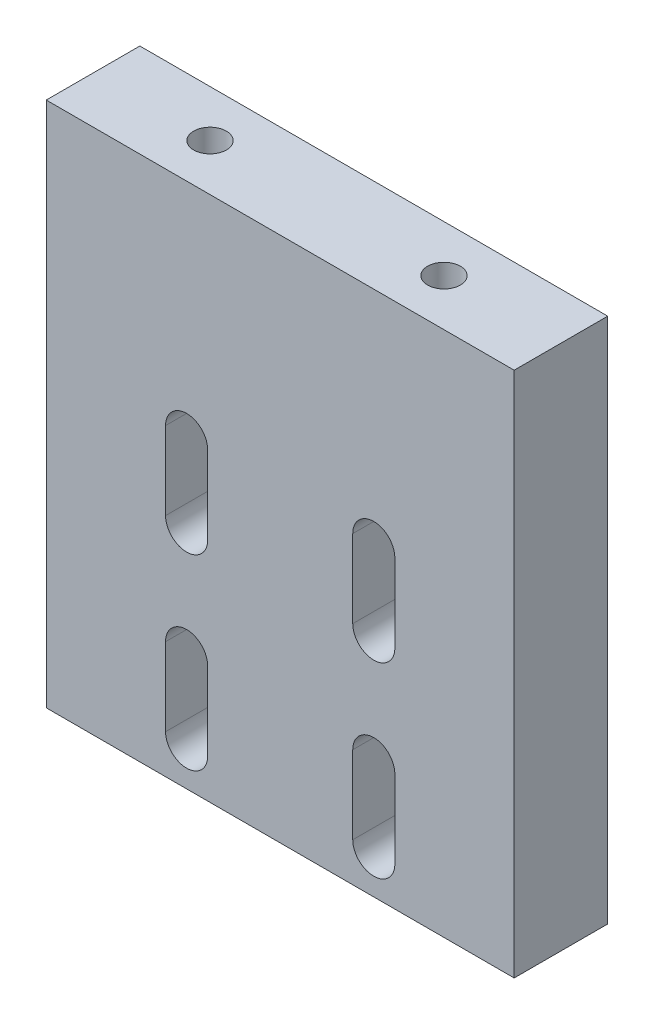
from build123d import *

# Parameters (mm, degrees)
SKETCH_1_W             = 60
SKETCH_1_H             = 67.5
EXTRUDE_1_DEPTH        = 6
CUT_EXTRUDE_1_DEPTH    = 47.723254382
HOLE_WIZARD_M5_1_D     = 4.2
HOLE_WIZARD_M5_1_DEPTH = 12.4
HOLE_WIZARD_M5_1_TIP   = 1.2618073


with BuildPart() as part:
    # 草图1 → 凸台-拉伸1 (new, symmetric)
    with BuildSketch(Plane.XY):
        Rectangle(SKETCH_1_W, SKETCH_1_H)
    extrude(amount=EXTRUDE_1_DEPTH, both=True)

    # 草图2 → 切除-拉伸1 (cut, through all)
    with BuildSketch(Plane(origin=(0, 0, -6), x_dir=(-1, 0, 0), z_dir=(0, 0, -1))):
        with BuildLine():
            Line((9.3, -28.75), (9.3, -18.75))
            ThreePointArc((9.3, -18.75), (12, -16.05), (14.7, -18.75))
            Line((14.7, -18.75), (14.7, -28.75))
            ThreePointArc((14.7, -28.75), (12, -31.45), (9.3, -28.75))
        make_face()
        with BuildLine():
            Line((-14.7, -28.75), (-14.7, -18.75))
            ThreePointArc((-14.7, -18.75), (-12, -16.05), (-9.3, -18.75))
            Line((-9.3, -18.75), (-9.3, -28.75))
            ThreePointArc((-9.3, -28.75), (-12, -31.45), (-14.7, -28.75))
        make_face()
        with BuildLine():
            Line((14.7, 5.25), (14.7, -4.75))
            ThreePointArc((14.7, -4.75), (12, -7.45), (9.3, -4.75))
            Line((9.3, -4.75), (9.3, 5.25))
            ThreePointArc((9.3, 5.25), (12, 7.95), (14.7, 5.25))
        make_face()
        with BuildLine():
            Line((-9.3, 5.25), (-9.3, -4.75))
            ThreePointArc((-9.3, -4.75), (-12, -7.45), (-14.7, -4.75))
            Line((-14.7, -4.75), (-14.7, 5.25))
            ThreePointArc((-14.7, 5.25), (-12, 7.95), (-9.3, 5.25))
        make_face()
    extrude(amount=-CUT_EXTRUDE_1_DEPTH, mode=Mode.SUBTRACT)

    # M5 螺纹孔1
    with Locations(Plane(origin=(0, 33.75, 0), x_dir=(1, 0, 0), z_dir=(0, 1, 0))):
        with Locations((-15, 0), (15, 0)):
            Hole(HOLE_WIZARD_M5_1_D / 2, depth=HOLE_WIZARD_M5_1_DEPTH)
            with Locations((0, 0, -(HOLE_WIZARD_M5_1_DEPTH + HOLE_WIZARD_M5_1_TIP / 2))):  # 118° drill point
                Cone(0, HOLE_WIZARD_M5_1_D / 2, HOLE_WIZARD_M5_1_TIP, mode=Mode.SUBTRACT)


solid = part.part
